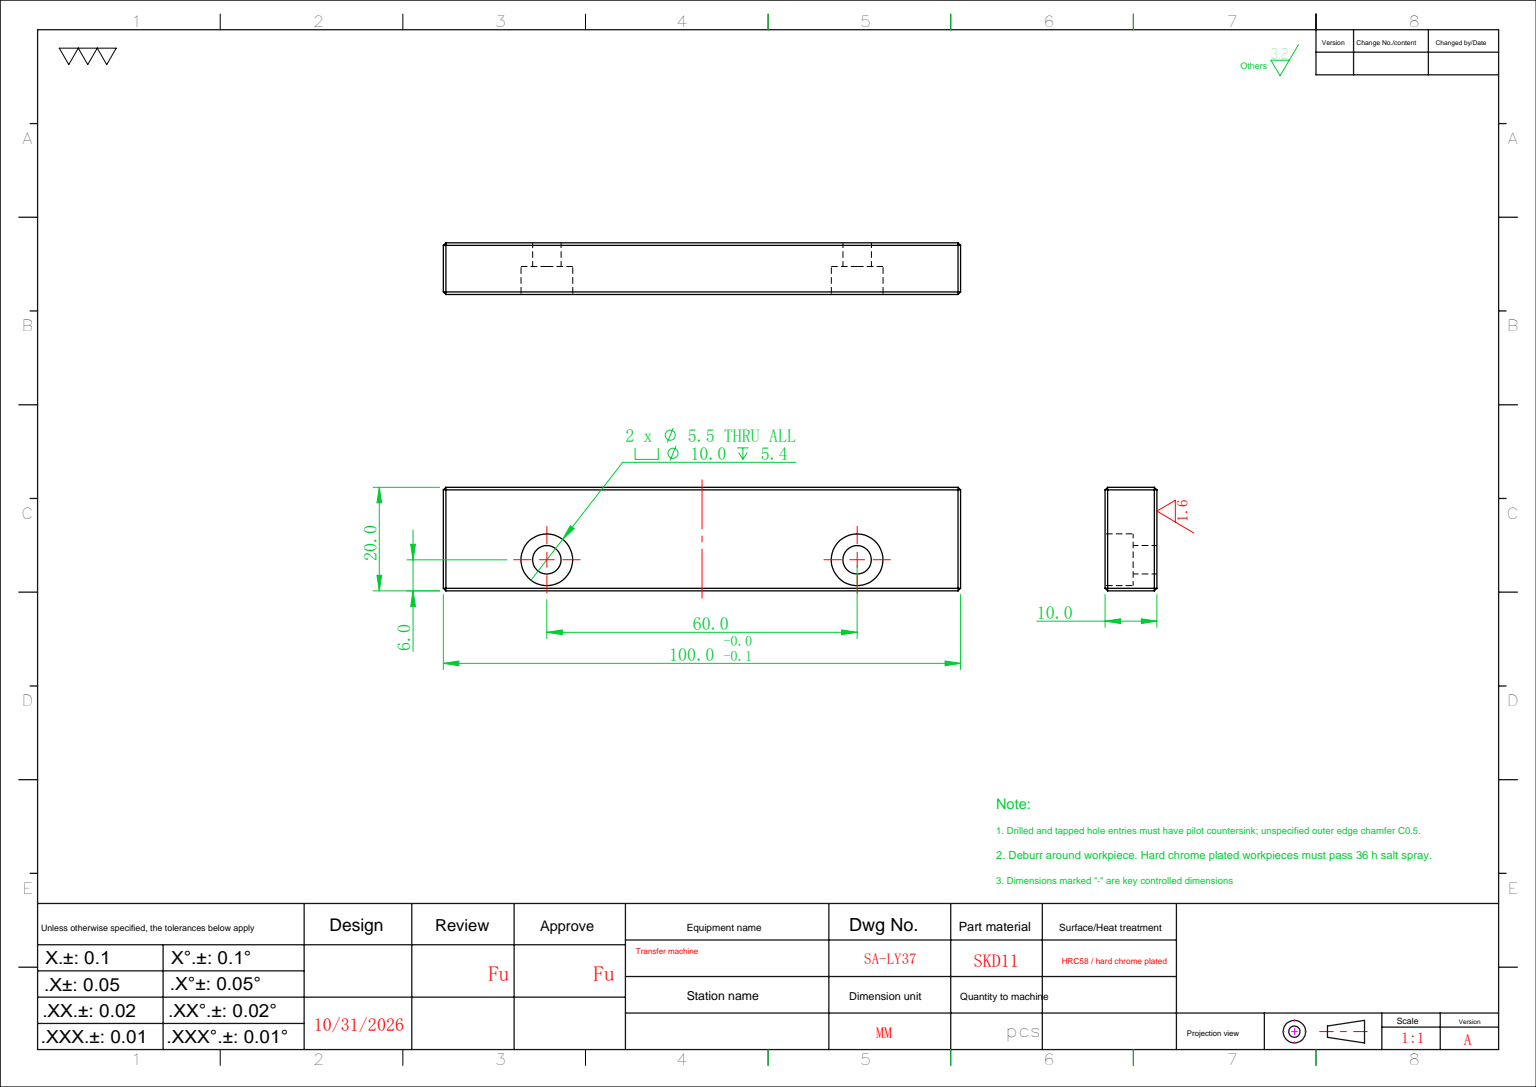
SolidWorks part; units mm, degrees
ref_plane "前视基准面" through (0, 0, 0) normal (0, 0, 1) x (1, 0, 0)
ref_plane "上视基准面" through (0, 0, 0) normal (0, 1, 0) x (1, 0, 0)
ref_plane "右视基准面" through (0, 0, 0) normal (1, 0, 0) x (0, 0, -1)
sketch "草图1" plane through (0, 0, 0) normal (0, 0, 1) x (1, 0, 0)
  line L1 (-5, -50) -> (5, -50)
  line L2 (-5, -50) -> (-5, 50)
  line L3 (-5, 50) -> (5, 50)
  line L4 (5, -50) -> (5, 50)
  line L5 (-5, -50) -> (5, 50) construction
  line L6 (-5, 50) -> (5, -50) construction
  point P0 (0, 0)
  dimension "D1" = 10
  dimension "D2" = 100
extrude "凸台-拉伸1" add sketch "草图1" along normal blind 20
hole_wizard "M5 六角凹头螺钉的柱形沉头孔1" positions "草图2" profile "草图3" counterbore size "M5" standard "ISO" end condition through all
sketch "草图2" plane through (-5, 0, 0) normal (-1, 0, 0) x (0, 0, 1)
  line L0 (0, 0) -> (32.9363, 0) construction
  line L2 (0, 50) -> (0, -50) construction
  point P0 (6, 30)
  point P2 (6, -30)
  dimension "D1" = 60
  dimension "D2" = 6
sketch "草图3" plane through (-5, 30, 6) normal (0, 1, 0) x (0, 0, 1)
  line L0 (0, 0) -> (0, 10)
  line L1 (0, 10) -> (2.75, 10)
  line L3 (2.75, 10) -> (2.75, 5.4)
  line L4 (2.75, 5.4) -> (5, 5.4)
  line L5 (5, 5.4) -> (5, 0)
  line L7 (5, 0) -> (0, 0)
  line L11 (0, -6.35) -> (0, 107.95) construction
  dimension "通孔孔直径" = 5.5
  dimension "通孔孔深度" = 10
  dimension "柱形沉头孔直径" = 10
  dimension "柱形沉头孔深度" = 5.4
chamfer "倒角1" distance 0.5 angle 45 12 edges at (5, 0, 20) (5, 0, 0) (-5, 0, 20) (-5, -50, 10) (0, -50, 20) (5, -50, 10) (0, -50, 0) (-5, 0, 0) (5, 50, 10) (0, 50, 20) (-5, 50, 10) (0, 50, 0)
